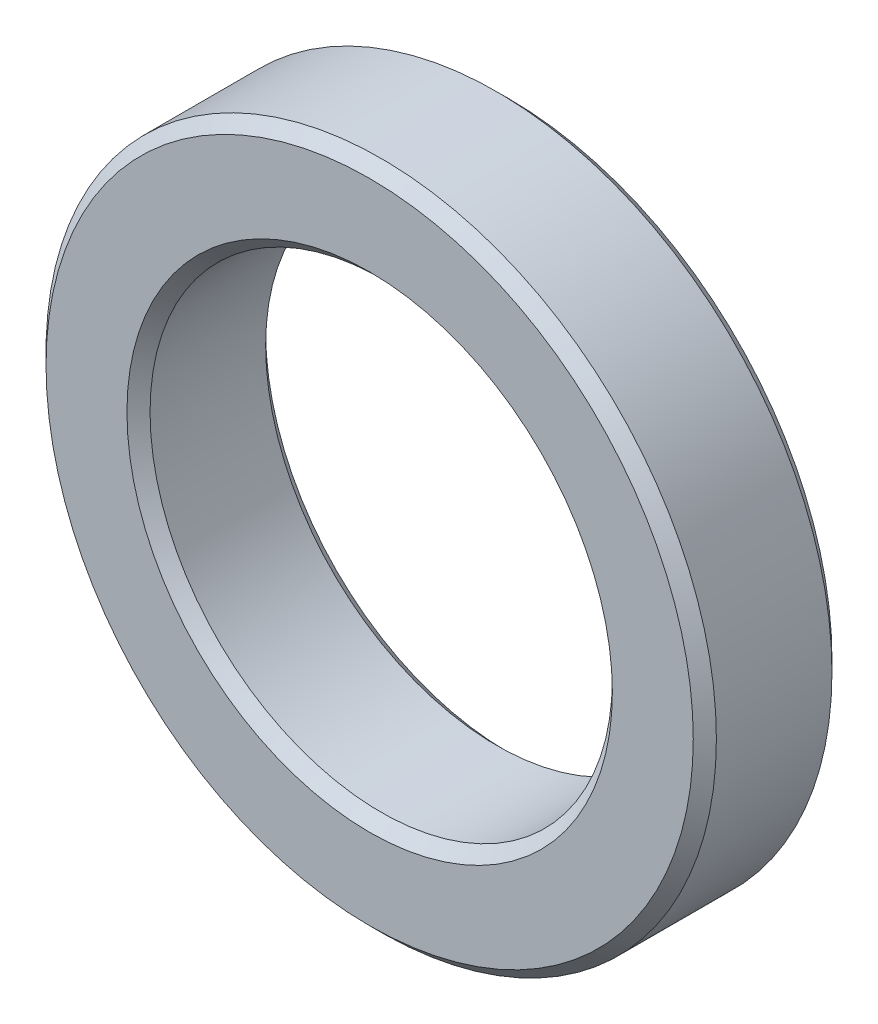
from build123d import *


with BuildPart() as part:
    # Sketch1 → Revolve1 (revolve)
    with BuildSketch(Plane(origin=(0, 0, 0), x_dir=(1, 0, 0), z_dir=(0, 1, 0))):
        Polygon((2.1, 0), (2.8, 0), (2.9, 0.1), (2.9, 1.1), (2.8, 1.2), (2.1, 1.2), (2, 1.1), (2, 0.1), align=None)
    revolve(axis=Axis((0, 0, 0), (0, 0, -1)))


solid = part.part
